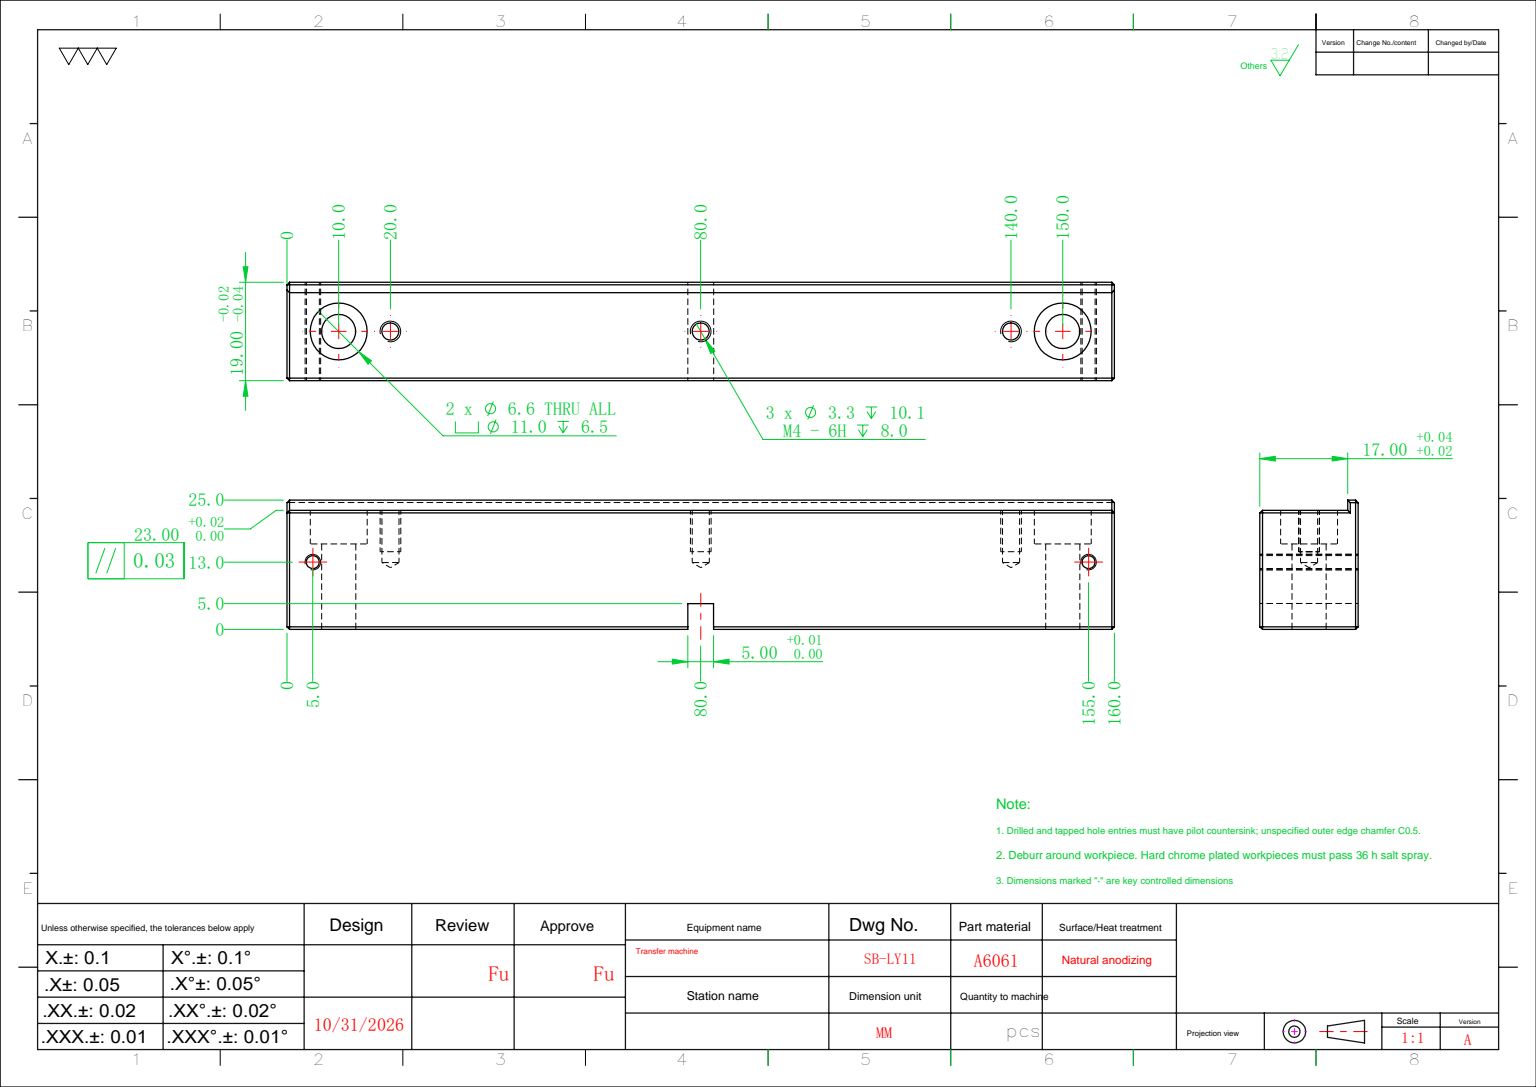
from build123d import *

# Parameters (mm, degrees)
SKETCH_1_W                   = 160
SKETCH_1_H                   = 25
EXTRUDE_1_DEPTH              = 19
SKETCH_2_W                   = 160
SKETCH_2_H                   = 15
CUT_EXTRUDE_1_DEPTH          = 2
HOLE_WIZARD_M4_1_D           = 3.3
HOLE_WIZARD_M4_1_DEPTH       = 10.1
HOLE_WIZARD_M4_1_TIP         = 0.991420021
HOLE_WIZARD_M6_1_D           = 6.6
HOLE_WIZARD_M6_1_CBORE_D     = 11
HOLE_WIZARD_M6_1_CBORE_DEPTH = 6.5
SKETCH_7_W                   = 5
SKETCH_7_H                   = 5
CUT_EXTRUDE_2_DEPTH          = 84.170006613
SKETCH_10_W                  = 2
SKETCH_10_H                  = 2
CUT_EXTRUDE_3_DEPTH          = 162.608322805
CHAMFER_1_SIZE               = 0.5
HOLE_WIZARD_M3_1_D           = 2.5


with BuildPart() as part:
    # 草图1 → 凸台-拉伸1 (new body)
    with BuildSketch(Plane.XY):
        Rectangle(SKETCH_1_W, SKETCH_1_H)
    extrude(amount=EXTRUDE_1_DEPTH)

    # 草图2 → 切除-拉伸1 (cut)
    with BuildSketch(Plane.XZ.offset(12.5)):
        with Locations((0, 9.5)):
            Rectangle(SKETCH_2_W, SKETCH_2_H)
    extrude(amount=-CUT_EXTRUDE_1_DEPTH, mode=Mode.SUBTRACT)

    # M4 螺纹孔1
    with Locations(Plane(origin=(0, -10.5, 0), x_dir=(-1, 0, 0), z_dir=(0, -1, 0))):
        with Locations((-60, -9.5), (0, -9.5), (60, -9.5)):
            Hole(HOLE_WIZARD_M4_1_D / 2, depth=HOLE_WIZARD_M4_1_DEPTH)
            with Locations((0, 0, -(HOLE_WIZARD_M4_1_DEPTH + HOLE_WIZARD_M4_1_TIP / 2))):  # 118° drill point
                Cone(0, HOLE_WIZARD_M4_1_D / 2, HOLE_WIZARD_M4_1_TIP, mode=Mode.SUBTRACT)

    # M6 六角凹头螺钉的柱形沉头孔1 (through all)
    with Locations(Plane(origin=(0, -10.5, 0), x_dir=(-1, 0, 0), z_dir=(0, -1, 0))):
        with Locations((-70, -9.5), (70, -9.5)):
            CounterBoreHole(HOLE_WIZARD_M6_1_D / 2, HOLE_WIZARD_M6_1_CBORE_D / 2, HOLE_WIZARD_M6_1_CBORE_DEPTH)

    # 草图7 → 切除-拉伸2 (cut, through all)
    with BuildSketch(Plane.XY.offset(19)):
        with Locations((0, 10)):
            Rectangle(SKETCH_7_W, SKETCH_7_H)
    extrude(amount=-CUT_EXTRUDE_2_DEPTH, mode=Mode.SUBTRACT)

    # 草图10 → 切除-拉伸3 (cut, through all)
    with BuildSketch(Plane(origin=(80, 0, 0), x_dir=(0, 0, -1), z_dir=(1, 0, 0))):
        with Locations((-18, -11.5)):
            Rectangle(SKETCH_10_W, SKETCH_10_H)
    extrude(amount=-CUT_EXTRUDE_3_DEPTH, mode=Mode.SUBTRACT)

    # 倒角1
    chamfer_1_edges = [part.edges().sort_by_distance(p)[0] for p in [
        (-80, 1, 19),
        (80, -12.5, 1),
        (-80, -12.5, 1),
        (80, -10.5, 10.5),
        (80, -11.5, 2),
        (-80, -10.5, 10.5),
        (-80, -11.5, 2),
        (0, -12.5, 0),
        (-80, 0, 0),
        (41.25, 12.5, 0),
        (80, 0, 0),
        (-41.25, 12.5, 0),
        (-41.25, 12.5, 19),
        (41.25, 12.5, 19),
        (-80, 12.5, 9.5),
        (80, 1, 19),
        (80, 12.5, 9.5),
        (0, -10.5, 19),
    ]]
    chamfer(chamfer_1_edges, length=CHAMFER_1_SIZE)

    # M3 螺纹孔1 (through all)
    with Locations(Plane.XY.offset(19)):
        with Locations((75, -0.5), (-75, -0.5)):
            Hole(HOLE_WIZARD_M3_1_D / 2)


solid = part.part
